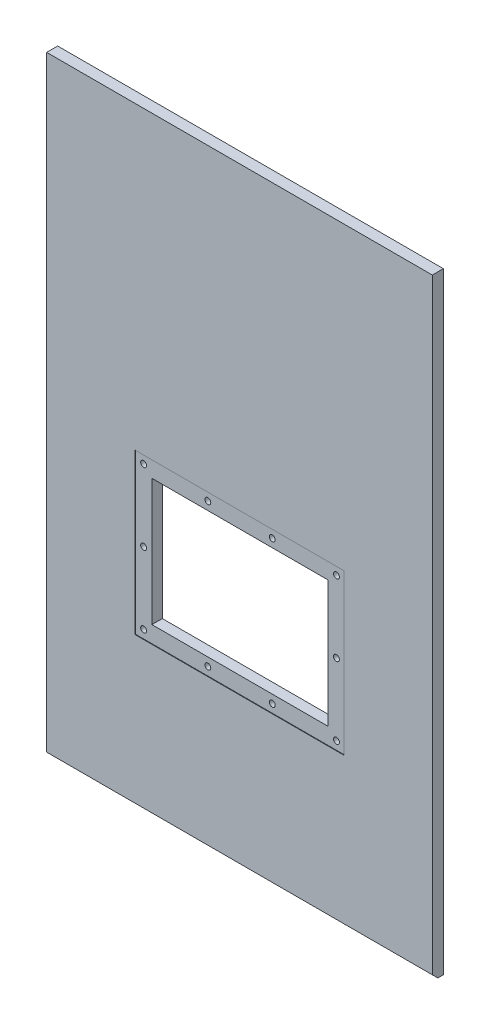
from build123d import *

# Parameters (mm, degrees)
SKETCH1_W                     = 700
SKETCH1_H                     = 1110
SKETCH1_W_2                   = 320
SKETCH1_H_2                   = 230
BOSS_EXTRUDE1_DEPTH           = 20
SKETCH2_W                     = 380
SKETCH2_H                     = 290
CUT_EXTRUDE1_DEPTH            = 1
F_1_2_13_THREADED_HOLE1_D     = 10.71626
F_1_2_13_THREADED_HOLE1_DEPTH = 14
F_1_2_13_THREADED_HOLE1_TIP   = 3.219489309
CHAMFER1_SIZE                 = 10


with BuildPart() as part:
    # Sketch1 → Boss-Extrude1 (new body)
    with BuildSketch(Plane.XY):
        with Locations((350, 555)):
            Rectangle(SKETCH1_W, SKETCH1_H)
        with Locations((350, 420)):
            Rectangle(SKETCH1_W_2, SKETCH1_H_2, mode=Mode.SUBTRACT)
    extrude(amount=BOSS_EXTRUDE1_DEPTH)

    # Sketch2 → Cut-Extrude1 (cut)
    with BuildSketch(Plane.XY.offset(20)):
        with Locations((350, 420)):
            Rectangle(SKETCH2_W, SKETCH2_H)
    extrude(amount=-CUT_EXTRUDE1_DEPTH, mode=Mode.SUBTRACT)

    # 1/2-13 Threaded hole1
    with Locations(Plane(origin=(175, 550, 19), x_dir=(1, 0, 0), z_dir=(0, 0, 1))):
        with Locations((0, 0), (116.5, 0), (233.5, 0), (350, 0), (350, -130), (350, -260), (233.5, -260), (116.5, -260), (0, -260), (0, -130)):
            Hole(F_1_2_13_THREADED_HOLE1_D / 2, depth=F_1_2_13_THREADED_HOLE1_DEPTH)
            with Locations((0, 0, -(F_1_2_13_THREADED_HOLE1_DEPTH + F_1_2_13_THREADED_HOLE1_TIP / 2))):  # 118° drill point
                Cone(0, F_1_2_13_THREADED_HOLE1_D / 2, F_1_2_13_THREADED_HOLE1_TIP, mode=Mode.SUBTRACT)

    # Chamfer1
    chamfer1_edges = [part.edges().sort_by_distance(p)[0] for p in [
        (350, 0, 20),
    ]]
    chamfer(chamfer1_edges, length=CHAMFER1_SIZE)


solid = part.part
